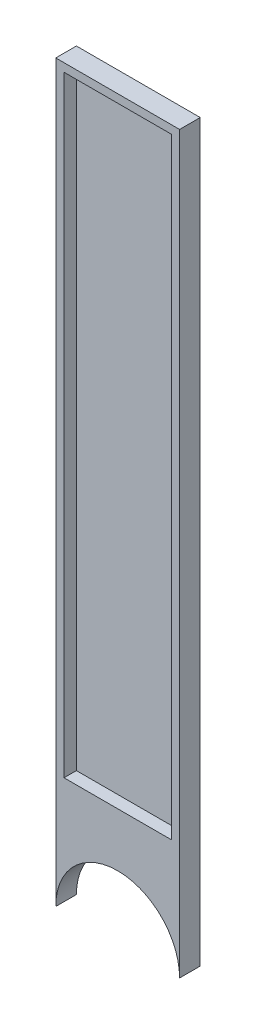
from build123d import *

# Parameters (mm, degrees)
SKETCH1_W           = 30
SKETCH1_H           = 178
BOSS_EXTRUDE1_DEPTH = 5
SKETCH3_W           = 26
SKETCH3_H           = 210
CUT_EXTRUDE1_DEPTH  = 3
SKETCH4_W           = 26
SKETCH4_H           = 10
BOSS_EXTRUDE2_DEPTH = 3
CUT_EXTRUDE3_DEPTH  = 5
BOSS_EXTRUDE3_START = 3
BOSS_EXTRUDE3_DEPTH = 3


with BuildPart() as part:
    # Sketch1 → Boss-Extrude1 (new body)
    with BuildSketch(Plane.XY):
        with Locations((15, 89)):
            Rectangle(SKETCH1_W, SKETCH1_H)
    extrude(amount=BOSS_EXTRUDE1_DEPTH)

    # Sketch3 → Cut-Extrude1 (cut)
    with BuildSketch(Plane.XY.offset(5)):
        with Locations((15, 71)):
            Rectangle(SKETCH3_W, SKETCH3_H)
    extrude(amount=-CUT_EXTRUDE1_DEPTH, mode=Mode.SUBTRACT)

    # Sketch4 → Boss-Extrude2 (add)
    with BuildSketch(Plane.XY.offset(2)):
        with Locations((15, 23)):
            Rectangle(SKETCH4_W, SKETCH4_H)
    extrude(amount=BOSS_EXTRUDE2_DEPTH)

    # Sketch5 → Cut-Extrude3 (cut, symmetric)
    with BuildSketch(Plane.XY.offset(2)):
        with BuildLine():
            Line((0, 0), (30, 0))
            ThreePointArc((30, 0), (15, 15), (0, 0))
        make_face()
    extrude(amount=CUT_EXTRUDE3_DEPTH, both=True, mode=Mode.SUBTRACT)

    # Sketch6 → Boss-Extrude3 (add)
    with BuildSketch(Plane.XY.offset(2).offset(BOSS_EXTRUDE3_START)):
        with BuildLine():
            Line((28, 7.483314774), (28, 18))
            Line((28, 18), (2, 18))
            Line((2, 18), (2, 7.483314774))
            ThreePointArc((2, 7.483314774), (15, 15), (28, 7.483314774))
        make_face()
    extrude(amount=-BOSS_EXTRUDE3_DEPTH)


solid = part.part
